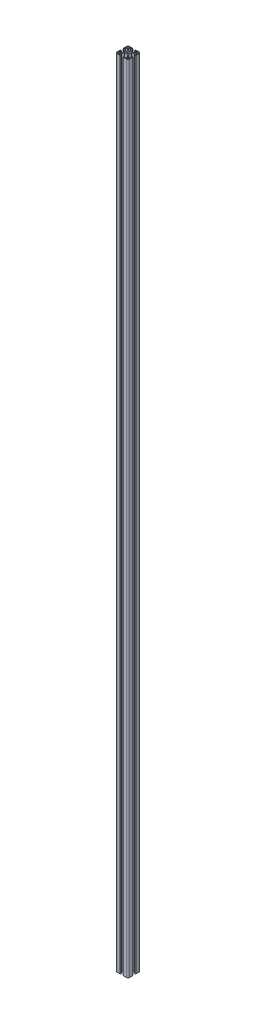
from build123d import *

# Parameters (mm, degrees)
SKETCH1_R                 = 3.4
F_40_X_40L_X_R4_5_1_DEPTH = 2550


with BuildPart() as part:
    # Sketch1 → 铝型材 40 X 40L X R4.5(1) (new body)
    with BuildSketch(Plane.ZX):
        with BuildLine():
            Line((-5.1, 20), (-5.1, 19.5))
            Line((-5.1, 19.5), (-4.1, 19.5))
            Line((-4.1, 19.5), (-4.1, 17))
            Line((-4.1, 17), (-6.1, 17))
            Line((-6.1, 17), (-6.1, 18.5))
            Line((-6.1, 18.5), (-10.3, 18.5))
            Line((-10.3, 18.5), (-10.3, 11.3))
            Line((-10.3, 11.3), (-5, 6))
            Line((-5, 6), (5, 6))
            Line((5, 6), (10.3, 11.3))
            Line((10.3, 11.3), (10.3, 18.5))
            Line((10.3, 18.5), (6.1, 18.5))
            Line((6.1, 18.5), (6.1, 17))
            Line((6.1, 17), (4.1, 17))
            Line((4.1, 17), (4.1, 19.5))
            Line((4.1, 19.5), (5.1, 19.5))
            Line((5.1, 19.5), (5.1, 20))
            Line((5.1, 20), (15.5, 20))
            ThreePointArc((15.5, 20), (18.681980515, 18.681980515), (20, 15.5))
            Line((20, 15.5), (20, 5.1))
            Line((20, 5.1), (19.5, 5.1))
            Line((19.5, 5.1), (19.5, 4.1))
            Line((19.5, 4.1), (17, 4.1))
            Line((17, 4.1), (17, 6.1))
            Line((17, 6.1), (18.5, 6.1))
            Line((18.5, 6.1), (18.5, 10.3))
            Line((18.5, 10.3), (11.3, 10.3))
            Line((11.3, 10.3), (6, 5))
            Line((6, 5), (6, -5))
            Line((6, -5), (11.3, -10.3))
            Line((11.3, -10.3), (18.5, -10.3))
            Line((18.5, -10.3), (18.5, -6.1))
            Line((18.5, -6.1), (17, -6.1))
            Line((17, -6.1), (17, -4.1))
            Line((17, -4.1), (19.5, -4.1))
            Line((19.5, -4.1), (19.5, -5.1))
            Line((19.5, -5.1), (20, -5.1))
            Line((20, -5.1), (20, -15.5))
            ThreePointArc((20, -15.5), (18.681980515, -18.681980515), (15.5, -20))
            Line((15.5, -20), (5.1, -20))
            Line((5.1, -20), (5.1, -19.5))
            Line((5.1, -19.5), (4.1, -19.5))
            Line((4.1, -19.5), (4.1, -17))
            Line((4.1, -17), (6.1, -17))
            Line((6.1, -17), (6.1, -18.5))
            Line((6.1, -18.5), (10.3, -18.5))
            Line((10.3, -18.5), (10.3, -11.3))
            Line((10.3, -11.3), (5, -6))
            Line((5, -6), (-5, -6))
            Line((-5, -6), (-10.3, -11.3))
            Line((-10.3, -11.3), (-10.3, -18.5))
            Line((-10.3, -18.5), (-6.1, -18.5))
            Line((-6.1, -18.5), (-6.1, -17))
            Line((-6.1, -17), (-4.1, -17))
            Line((-4.1, -17), (-4.1, -19.5))
            Line((-4.1, -19.5), (-5.1, -19.5))
            Line((-5.1, -19.5), (-5.1, -20))
            Line((-5.1, -20), (-15.5, -20))
            ThreePointArc((-15.5, -20), (-18.681980515, -18.681980515), (-20, -15.5))
            Line((-20, -15.5), (-20, -5.1))
            Line((-20, -5.1), (-19.5, -5.1))
            Line((-19.5, -5.1), (-19.5, -4.1))
            Line((-19.5, -4.1), (-17, -4.1))
            Line((-17, -4.1), (-17, -6.1))
            Line((-17, -6.1), (-18.5, -6.1))
            Line((-18.5, -6.1), (-18.5, -10.3))
            Line((-18.5, -10.3), (-11.3, -10.3))
            Line((-11.3, -10.3), (-6, -5))
            Line((-6, -5), (-6, 5))
            Line((-6, 5), (-11.3, 10.3))
            Line((-11.3, 10.3), (-18.5, 10.3))
            Line((-18.5, 10.3), (-18.5, 6.1))
            Line((-18.5, 6.1), (-17, 6.1))
            Line((-17, 6.1), (-17, 4.1))
            Line((-17, 4.1), (-19.5, 4.1))
            Line((-19.5, 4.1), (-19.5, 5.1))
            Line((-19.5, 5.1), (-20, 5.1))
            Line((-20, 5.1), (-20, 15.5))
            ThreePointArc((-20, 15.5), (-18.681980515, 18.681980515), (-15.5, 20))
            Line((-15.5, 20), (-5.1, 20))
        make_face()
        Circle(SKETCH1_R, mode=Mode.SUBTRACT)
        with BuildLine():
            Line((11.8, 17.5), (15, 17.5))
            ThreePointArc((15, 17.5), (16.767766953, 16.767766953), (17.5, 15))
            Line((17.5, 15), (17.5, 11.8))
            Line((17.5, 11.8), (11.8, 11.8))
            Line((11.8, 11.8), (11.8, 17.5))
        make_face(mode=Mode.SUBTRACT)
        with BuildLine():
            Line((-15, 17.5), (-11.8, 17.5))
            Line((-11.8, 17.5), (-11.8, 11.8))
            Line((-11.8, 11.8), (-17.5, 11.8))
            Line((-17.5, 11.8), (-17.5, 15))
            ThreePointArc((-17.5, 15), (-16.767766953, 16.767766953), (-15, 17.5))
        make_face(mode=Mode.SUBTRACT)
        with BuildLine():
            Line((-17.5, -11.8), (-11.8, -11.8))
            Line((-11.8, -11.8), (-11.8, -17.5))
            Line((-11.8, -17.5), (-15, -17.5))
            ThreePointArc((-15, -17.5), (-16.767766953, -16.767766953), (-17.5, -15))
            Line((-17.5, -15), (-17.5, -11.8))
        make_face(mode=Mode.SUBTRACT)
        with BuildLine():
            Line((11.8, -11.8), (17.5, -11.8))
            Line((17.5, -11.8), (17.5, -15))
            ThreePointArc((17.5, -15), (16.767766953, -16.767766953), (15, -17.5))
            Line((15, -17.5), (11.8, -17.5))
            Line((11.8, -17.5), (11.8, -11.8))
        make_face(mode=Mode.SUBTRACT)
    extrude(amount=F_40_X_40L_X_R4_5_1_DEPTH)


solid = part.part
